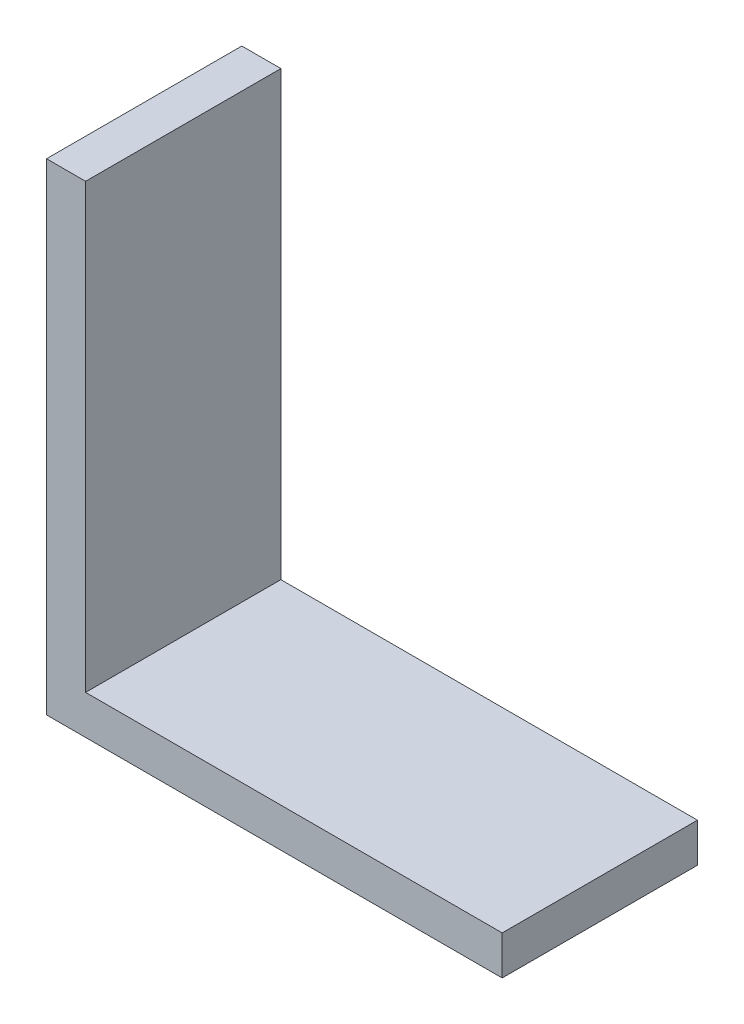
from build123d import *

# Parameters (mm, degrees)
EXTRUDE_1_DEPTH = 15


with BuildPart() as part:
    # 草图1 → 凸台-拉伸1 (new, symmetric)
    with BuildSketch(Plane.XY):
        Polygon((0, 0), (70, 0), (70, 6), (6, 6), (6, 74), (0, 74), align=None)
    extrude(amount=EXTRUDE_1_DEPTH, both=True)


solid = part.part
